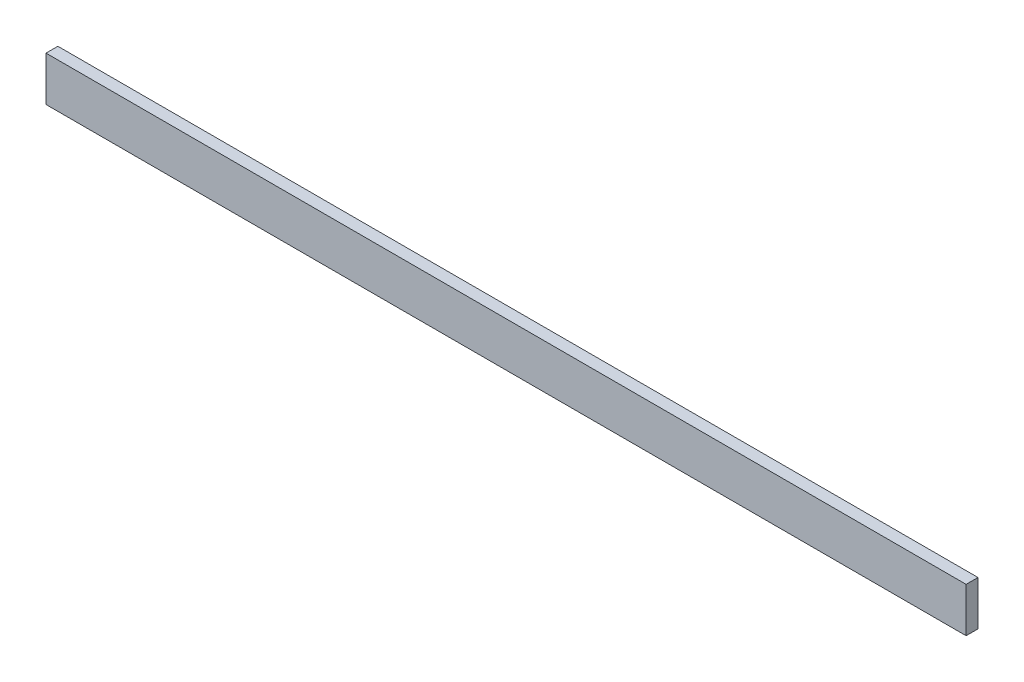
from build123d import *

# Parameters (mm, degrees)
SKETCH1_W           = 620
SKETCH1_H           = 30
BOSS_EXTRUDE1_DEPTH = 8


with BuildPart() as part:
    # Sketch1 → Boss-Extrude1 (new body)
    with BuildSketch(Plane.XY):
        with Locations((310, 15)):
            Rectangle(SKETCH1_W, SKETCH1_H)
    extrude(amount=BOSS_EXTRUDE1_DEPTH)


solid = part.part
